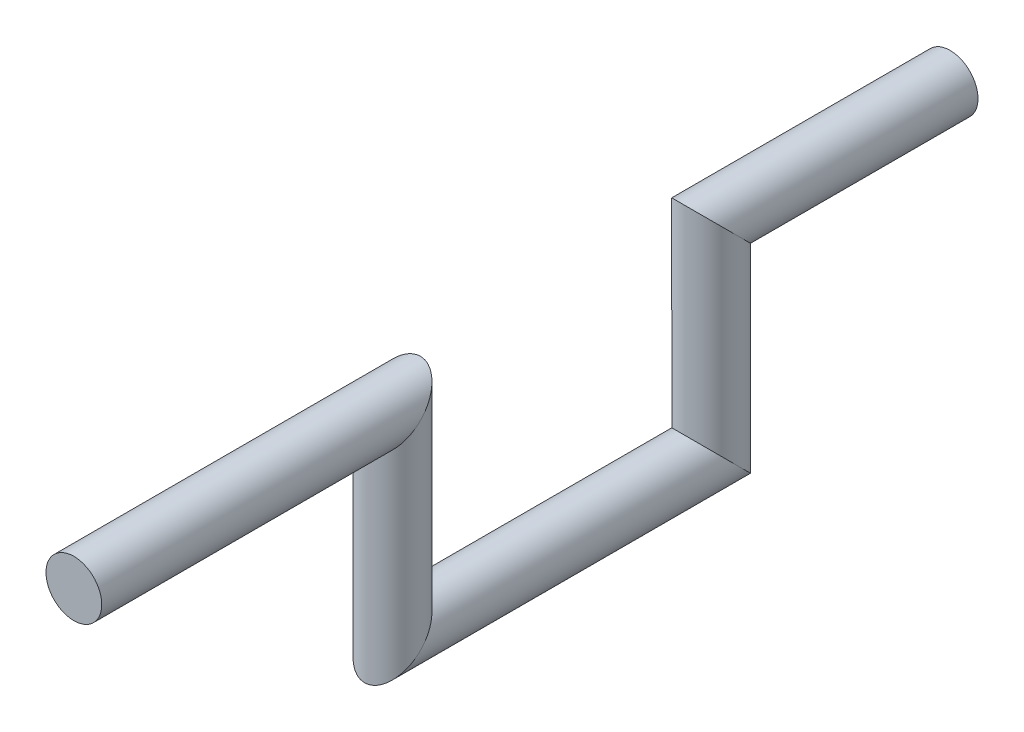
from build123d import *

# Parameters (mm, degrees)
SKETCH_1_R = 7


with BuildPart() as part:
    # 扫描1: sweep along a path in 草图3
    with BuildLine(Plane(origin=(0, 0, 0), x_dir=(0, 0, -1), z_dir=(1, 0, 0))) as sweep_1_path:
        Line((0, 0), (80, 0))
        Line((80, 0), (80, -50))
        Line((80, -50), (160, -50))
        Line((160, -50), (160, 0))
        Line((160, 0), (220, 0))
    # 草图1 → 扫描1 (sweep)
    with BuildSketch(Plane.XY):
        Circle(SKETCH_1_R)
    sweep(path=sweep_1_path.line, transition=Transition.RIGHT)


solid = part.part
